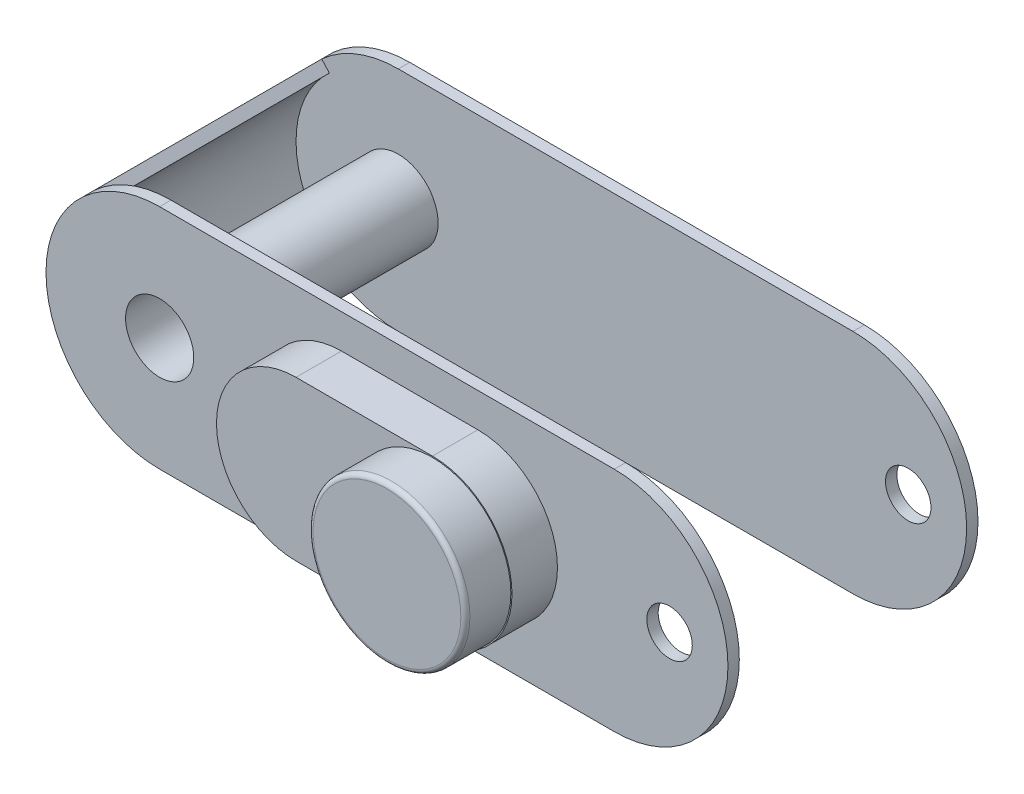
SolidWorks part; units mm, degrees
ref_plane "Front Plane" through (0, 0, 0) normal (0, 0, 1) x (1, 0, 0)
ref_plane "Top Plane" through (0, 0, 0) normal (0, 1, 0) x (1, 0, 0)
ref_plane "Right Plane" through (0, 0, 0) normal (1, 0, 0) x (0, 0, -1)
other "Configuration Table"
sketch "Sketch5" plane through (0, 0, 0) normal (0, 0, 1) x (1, 0, 0)
  line L0 (50, 0) -> (100, 0) construction
  line L1 (0, 50) -> (200, 50)
  line L2 (0, -50) -> (200, -50)
  arc A0 (0, 50) -> (0, -50) centre (0, 0) ccw
  arc A1 (200, -50) -> (200, 50) centre (200, 0) ccw
  circle A2 centre (0, 0) radius 15
  dimension "D1" = 100
  dimension "D3" = 30
  dimension "D2" = 200
extrude "Boss-Extrude2" add sketch "Sketch5" along normal blind 5
sketch "Sketch6" plane through (0, 0, 5) normal (0, 0, 1) x (1, 0, 0)
  line L2 (0, -50) -> (200, -50)
  line L3 (200, 50) -> (0, 50)
  line L4 (0, -50) -> (200, -50)
  line L5 (200, 50) -> (0, 50)
  circle A0 centre (0, 0) radius 15 construction
  circle A1 centre (0, 0) radius 15
  arc A2 (0, 50) -> (0, -50) centre (0, 0) ccw
  arc A3 (200, -50) -> (200, 50) centre (200, 0) ccw
  arc A4 (0, 50) -> (0, -50) centre (0, 0) ccw
  arc A5 (200, -50) -> (200, 50) centre (200, 0) ccw
  dimension "D1" = 0
extrude "Boss-Extrude3" add sketch "Sketch6" along normal blind 5 from offset 100 separate body
sketch "Sketch7" plane through (0, 0, 5) normal (0, 0, 1) x (1, 0, 0)
  circle A0 centre (0, 0) radius 15 construction
  circle A1 centre (0, 0) radius 15
  circle A2 centre (0, 0) radius 17.5
  dimension "D1" = 35
extrude "Boss-Extrude4" add sketch "Sketch7" along normal up to surface (100 mm away) up to face at (100, 0, 105)
sketch "Sketch8" plane through (0, 0, 105) normal (0, 0, -1) x (-1, 0, 0)
  line L0 (-140, 0) -> (-80, 0) construction
  circle A0 centre (-80, 0) radius 10
  circle A1 centre (-140, 0) radius 10
  dimension "D1" = 20
  dimension "D2" = 20
  dimension "D3" = 60
  dimension "D4" = 80
extrude "Cut-Extrude1" cut sketch "Sketch8" against normal blind 46 contours A1 | A0
sketch "Sketch9" plane through (0, 0, 110) normal (0, 0, 1) x (1, 0, 0)
  line L0 (80, 0) -> (140, 0) construction
  line L1 (80, 35) -> (140, 35)
  line L2 (80, -35) -> (140, -35)
  arc A0 (80, 35) -> (80, -35) centre (80, 0) ccw
  arc A1 (140, -35) -> (140, 35) centre (140, 0) ccw
  point P4 (110, 0)
  dimension "D1" = 70
extrude "Boss-Extrude5" add sketch "Sketch9" along normal blind 20
sketch "Sketch10" plane through (0, 0, 130) normal (0, 0, 1) x (1, 0, 0)
  circle A0 centre (140, 0) radius 34.5
  dimension "D1" = 69
extrude "Boss-Extrude6" add sketch "Sketch10" along normal blind 20
sketch "Sketch11" plane through (0, 0, 0) normal (0, 0, -1) x (-1, 0, 0)
  circle A0 centre (-224.3074, 0) radius 10
  dimension "D1" = 20
extrude "Cut-Extrude2" cut sketch "Sketch11" against normal blind 127
sketch "Sketch13" plane through (0, 0, 5) normal (0, 0, 1) x (1, 0, 0)
  line L2 (0, -50) -> (200, -50)
  line L3 (200, 50) -> (0, 50)
  line L6 (-33.7131, 36.9246) -> (-30.3418, 33.2321)
  line L7 (-40.0397, -29.947) -> (-36.0357, -26.9523)
  line L8 (0, -45) -> (200, -45)
  line L9 (200, 45) -> (0, 45)
  arc A2 (0, 50) -> (0, -50) centre (0, 0) ccw
  arc A3 (200, -50) -> (200, 50) centre (200, 0) ccw
  arc A4 (-33.7131, 36.9246) -> (-40.0397, -29.947) centre (0, 0) ccw
  arc A8 (0, 45) -> (0, -45) centre (0, 0) ccw
  arc A9 (200, -45) -> (200, 45) centre (200, 0) ccw
  arc A10 (-30.3418, 33.2321) -> (-36.0357, -26.9523) centre (0, 0) ccw
  dimension "D1" = 0
  dimension "D2" = 5
extrude "Boss-Extrude8" add sketch "Sketch13" along normal up to next
fillet "Fillet1" radius 2 1 edges at (174.5, 0, 150)
